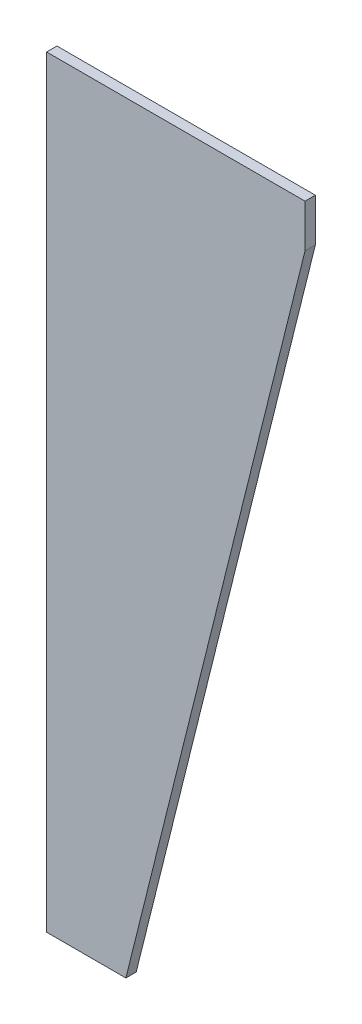
from build123d import *

# Parameters (mm, degrees)
BOSS_EXTRUDE1_DEPTH = 12


with BuildPart() as part:
    # Sketch1 → Boss-Extrude1 (new body)
    with BuildSketch(Plane.XY):
        Polygon((0, 0), (0, 885), (300, 885), (300, 835), (92, 0), align=None)
    extrude(amount=BOSS_EXTRUDE1_DEPTH)


solid = part.part
